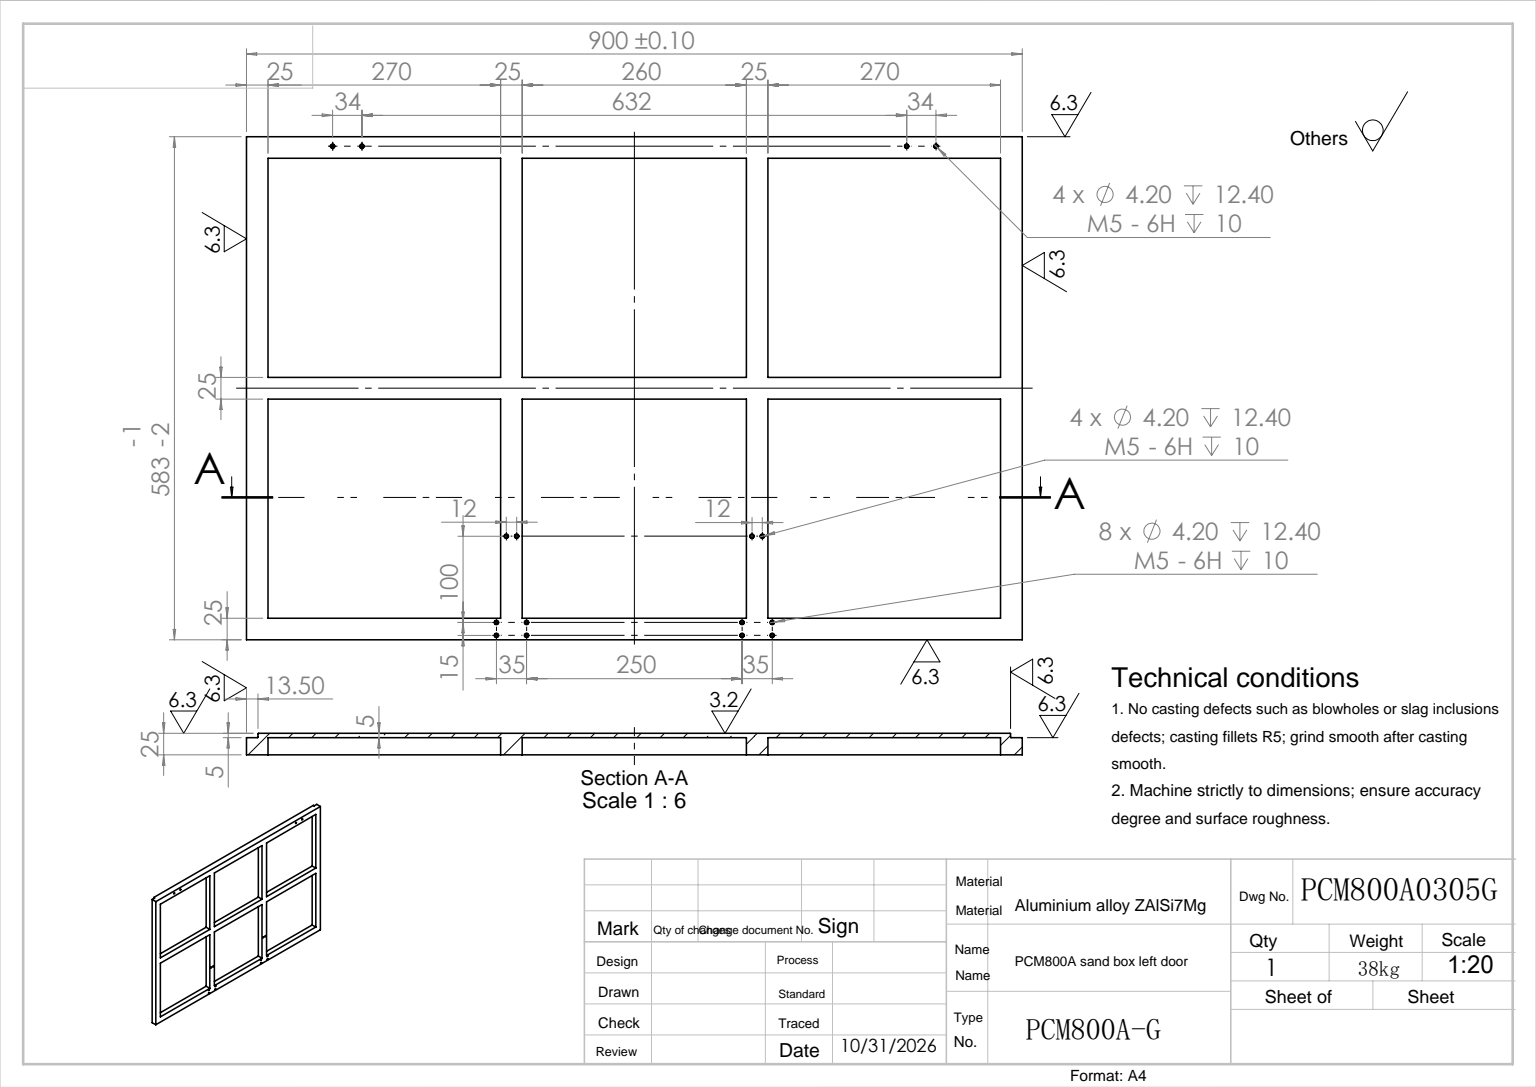
from build123d import *

# Parameters (mm, degrees)
SKETCH_1_W                  = 900
SKETCH_1_H                  = 583
EXTRUDE_1_DEPTH             = 5
SKETCH_2_W                  = 25
SKETCH_2_H                  = 583
EXTRUDE_2_DEPTH             = 20
SKETCH_3_W                  = 850
SKETCH_3_H                  = 25
EXTRUDE_3_DEPTH             = 20
SKETCH_4_W                  = 850
SKETCH_4_H                  = 25
EXTRUDE_4_DEPTH             = 20
SKETCH_5_W                  = 25
SKETCH_5_H                  = 533
EXTRUDE_5_DEPTH             = 20
SKETCH_6_W                  = 5
SKETCH_6_H                  = 13.5
CUT_EXTRUDE_1_DEPTH         = 1073.620156439
CHAMFER_1_SIZE              = 0.5
SKETCH_7_W                  = 5
SKETCH_7_H                  = 13.5
CUT_EXTRUDE_2_DEPTH         = 1073.620156439
CHAMFER_2_SIZE              = 0.5
PATTERN_LINEAR_1_COUNT      = 2
PATTERN_LINEAR_1_PITCH      = 35
PATTERN_LINEAR_1_COUNT_DIR2 = 2
PATTERN_LINEAR_1_PITCH_DIR2 = 15
HOLE_WIZARD_M5_2_AT_2_COUNT = 2
HOLE_WIZARD_M5_2_AT_2_PITCH = 12
PATTERN_LINEAR_2_COUNT      = 2
PATTERN_LINEAR_2_PITCH      = 285
HOLE_WIZARD_M5_3_AT_2_COUNT = 2
HOLE_WIZARD_M5_3_AT_2_PITCH = 34
PATTERN_LINEAR_3_COUNT      = 2
PATTERN_LINEAR_3_PITCH      = 666


with BuildPart() as part:
    # 草图1 → 拉伸1 (new body)
    with BuildSketch(Plane(origin=(0, 0, 0), x_dir=(0, 0, -1), z_dir=(1, 0, 0))):
        with Locations((450, 291.5)):
            Rectangle(SKETCH_1_W, SKETCH_1_H)
    extrude(amount=EXTRUDE_1_DEPTH)

    # 草图2 → 拉伸2 (add)
    with BuildSketch(Plane(origin=(5, 0, 0), x_dir=(0, 0, -1), z_dir=(1, 0, 0))):
        with Locations((12.5, 291.5)):
            Rectangle(SKETCH_2_W, SKETCH_2_H)
        with Locations((887.5, 291.5)):
            Rectangle(SKETCH_2_W, SKETCH_2_H)
    extrude(amount=EXTRUDE_2_DEPTH)

    # 草图3 → 拉伸3 (add)
    with BuildSketch(Plane(origin=(5, 0, 0), x_dir=(0, 0, -1), z_dir=(1, 0, 0))):
        with Locations((450, 570.5)):
            Rectangle(SKETCH_3_W, SKETCH_3_H)
        with Locations((450, 12.5)):
            Rectangle(SKETCH_3_W, SKETCH_3_H)
    extrude(amount=EXTRUDE_3_DEPTH)

    # 草图4 → 拉伸4 (add)
    with BuildSketch(Plane(origin=(5, 0, 0), x_dir=(0, 0, -1), z_dir=(1, 0, 0))):
        with Locations((450, 291.5)):
            Rectangle(SKETCH_4_W, SKETCH_4_H)
    extrude(amount=EXTRUDE_4_DEPTH)

    # 草图5 → 拉伸5 (add)
    with BuildSketch(Plane(origin=(5, 0, 0), x_dir=(0, 0, -1), z_dir=(1, 0, 0))):
        with Locations((307.5, 291.5)):
            Rectangle(SKETCH_5_W, SKETCH_5_H)
        with Locations((592.5, 291.5)):
            Rectangle(SKETCH_5_W, SKETCH_5_H)
    extrude(amount=EXTRUDE_5_DEPTH)

    # 草图6 → 切除-拉伸1 (cut, through all)
    with BuildSketch(Plane(origin=(0, 583, 0), x_dir=(-1, 0, 0), z_dir=(0, 1, 0))):
        with Locations((-2.5, -6.75)):
            Rectangle(SKETCH_6_W, SKETCH_6_H)
    extrude(amount=-CUT_EXTRUDE_1_DEPTH, mode=Mode.SUBTRACT)

    # 倒角1
    chamfer_1_edges = [part.edges().sort_by_distance(p)[0] for p in [
        (0, 291.5, -13.5),
        (5, 291.5, -13.5),
    ]]
    chamfer(chamfer_1_edges, length=CHAMFER_1_SIZE)

    # 草图7 → 切除-拉伸2 (cut, through all)
    with BuildSketch(Plane(origin=(0, 583, 0), x_dir=(-1, 0, 0), z_dir=(0, 1, 0))):
        with Locations((-2.5, -893.25)):
            Rectangle(SKETCH_7_W, SKETCH_7_H)
    extrude(amount=-CUT_EXTRUDE_2_DEPTH, mode=Mode.SUBTRACT)

    # 倒角2
    chamfer_2_edges = [part.edges().sort_by_distance(p)[0] for p in [
        (0, 291.5, -886.5),
        (5, 291.5, -886.5),
    ]]
    chamfer(chamfer_2_edges, length=CHAMFER_2_SIZE)

    # 草图8 → M5 螺纹孔1 (revolve, cut)
    with BuildSketch(Plane(origin=(25, 5, -290), x_dir=(0, 0, -1), z_dir=(0, 1, 0))):
        Polygon((0, 0), (0, 13.6618073), (2.1, 12.4), (2.1, 10), (2.5, 10), (2.5, 0), align=None)
    hole_wizard_m5_1 = revolve(axis=Axis((31.35, 5, -290), (-1, 0, 0)), mode=Mode.SUBTRACT)

    # 阵列(线性)1: Hole Wizard M5 _1 2 × 2
    with Locations(*[(0, j * PATTERN_LINEAR_1_PITCH_DIR2, -i * PATTERN_LINEAR_1_PITCH) for i in range(PATTERN_LINEAR_1_COUNT) for j in range(PATTERN_LINEAR_1_COUNT_DIR2) if (i, j) != (0, 0)]):
        add(hole_wizard_m5_1, mode=Mode.SUBTRACT)

    # 草图9 → M5 螺纹孔2 (revolve, cut)
    with BuildSketch(Plane(origin=(25, 120, -301.5), x_dir=(0, 0, -1), z_dir=(0, 1, 0))):
        Polygon((0, 0), (0, 13.6618073), (2.1, 12.4), (2.1, 10), (2.5, 10), (2.5, 0), align=None)
    hole_wizard_m5_2 = revolve(axis=Axis((31.35, 120, -301.5), (-1, 0, 0)), mode=Mode.SUBTRACT)

    # M5 螺纹孔2 at 2: M5 螺纹孔2 ×2
    with Locations(*[(0, 0, -i * HOLE_WIZARD_M5_2_AT_2_PITCH) for i in range(1, HOLE_WIZARD_M5_2_AT_2_COUNT)]):
        add(hole_wizard_m5_2, mode=Mode.SUBTRACT)

    # 阵列(线性)2: M5 螺纹孔1, M5 螺纹孔2 ×2
    with Locations(*[(0, 0, -i * PATTERN_LINEAR_2_PITCH) for i in range(1, PATTERN_LINEAR_2_COUNT)]):
        add(hole_wizard_m5_1, mode=Mode.SUBTRACT)
        add(hole_wizard_m5_2, mode=Mode.SUBTRACT)

    # 阵列(线性)2 copy 1 sketch → 阵列(线性)2 copy 1 (revolve, cut)
    with BuildSketch(Plane(origin=(25, 20, -575), x_dir=(0, 0, -1), z_dir=(0, 1, 0))):
        Polygon((0, 0), (0, 13.6618073), (2.1, 12.4), (2.1, 10), (2.5, 10), (2.5, 0), align=None)
    revolve(axis=Axis((31.35, 20, -575), (-1, 0, 0)), mode=Mode.SUBTRACT)

    # 阵列(线性)2 copy 2 sketch → 阵列(线性)2 copy 2 (revolve, cut)
    with BuildSketch(Plane(origin=(25, 5, -610), x_dir=(0, 0, -1), z_dir=(0, 1, 0))):
        Polygon((0, 0), (0, 13.6618073), (2.1, 12.4), (2.1, 10), (2.5, 10), (2.5, 0), align=None)
    revolve(axis=Axis((31.35, 5, -610), (-1, 0, 0)), mode=Mode.SUBTRACT)

    # 阵列(线性)2 copy 3 sketch → 阵列(线性)2 copy 3 (revolve, cut)
    with BuildSketch(Plane(origin=(25, 20, -610), x_dir=(0, 0, -1), z_dir=(0, 1, 0))):
        Polygon((0, 0), (0, 13.6618073), (2.1, 12.4), (2.1, 10), (2.5, 10), (2.5, 0), align=None)
    revolve(axis=Axis((31.35, 20, -610), (-1, 0, 0)), mode=Mode.SUBTRACT)

    # 阵列(线性)2 copy 4 sketch → 阵列(线性)2 copy 4 (revolve, cut)
    with BuildSketch(Plane(origin=(25, 120, -598.5), x_dir=(0, 0, -1), z_dir=(0, 1, 0))):
        Polygon((0, 0), (0, 13.6618073), (2.1, 12.4), (2.1, 10), (2.5, 10), (2.5, 0), align=None)
    revolve(axis=Axis((31.35, 120, -598.5), (-1, 0, 0)), mode=Mode.SUBTRACT)

    # 草图10 → M5 螺纹孔3 (revolve, cut)
    with BuildSketch(Plane(origin=(25, 572, -100), x_dir=(0, 0, -1), z_dir=(0, 1, 0))):
        Polygon((0, 0), (0, 13.6618073), (2.1, 12.4), (2.1, 10), (2.5, 10), (2.5, 0), align=None)
    hole_wizard_m5_3 = revolve(axis=Axis((31.35, 572, -100), (-1, 0, 0)), mode=Mode.SUBTRACT)

    # M5 螺纹孔3 at 2: M5 螺纹孔3 ×2
    with Locations(*[(0, 0, -i * HOLE_WIZARD_M5_3_AT_2_PITCH) for i in range(1, HOLE_WIZARD_M5_3_AT_2_COUNT)]):
        add(hole_wizard_m5_3, mode=Mode.SUBTRACT)

    # 阵列(线性)3: M5 螺纹孔3 ×2
    with Locations(*[(0, 0, -i * PATTERN_LINEAR_3_PITCH) for i in range(1, PATTERN_LINEAR_3_COUNT)]):
        add(hole_wizard_m5_3, mode=Mode.SUBTRACT)

    # 阵列(线性)3 copy 1 sketch → 阵列(线性)3 copy 1 (revolve, cut)
    with BuildSketch(Plane(origin=(25, 572, -800), x_dir=(0, 0, -1), z_dir=(0, 1, 0))):
        Polygon((0, 0), (0, 13.6618073), (2.1, 12.4), (2.1, 10), (2.5, 10), (2.5, 0), align=None)
    revolve(axis=Axis((31.35, 572, -800), (-1, 0, 0)), mode=Mode.SUBTRACT)


solid = part.part
